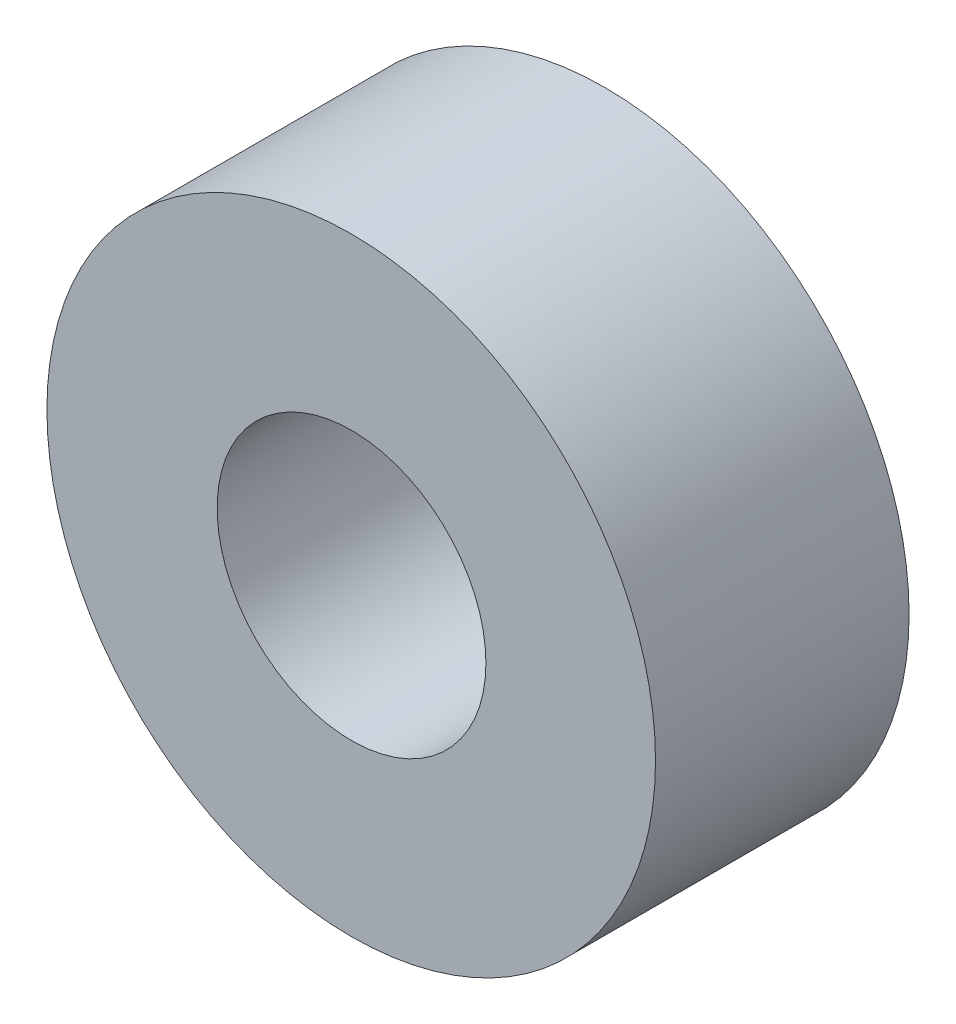
SolidWorks part; units mm, degrees
ref_plane "Front Plane" through (0, 0, 0) normal (0, 0, 1) x (1, 0, 0)
ref_plane "Top Plane" through (0, 0, 0) normal (0, 1, 0) x (1, 0, 0)
ref_plane "Right Plane" through (0, 0, 0) normal (1, 0, 0) x (0, 0, -1)
sketch "Sketch1" plane through (0, 0, 0) normal (0, 0, 1) x (1, 0, 0)
  circle A1 centre (0, 0) radius 30
extrude "Boss-Extrude1" add sketch "Sketch1" along normal blind 25
sketch "Sketch4" plane through (0, 0, 25) normal (0, 0, 1) x (1, 0, 0)
  circle A0 centre (0, 0) radius 13.2823
hole_wizard "M30 Tapped Hole3" positions "3DSketch4" profile "Sketch9" tap size "M30" standard "Gb"
sketch3d "3DSketch4"
  point P0 (0, 0, 0)
  point P3 (0.0315, -0.0033, 25)
sketch "Sketch9" plane through (0.0315, -0.0033, 25) normal (1, 0, 0) x (0, -1, 0)
  line L0 (0, 0) -> (0, 78.4614)
  line L1 (0, 78.4614) -> (13.25, 70.5)
  line L2 (13.25, 70.5) -> (13.25, 0)
  line L5 (13.25, 0) -> (0, 0)
  line L10 (0, 78.4614) -> (-13.25, 70.5) construction
  line L11 (0, -6.35) -> (0, 107.95) construction
  dimension "螺纹孔钻头直径" = 26.5
  dimension "螺纹孔钻头深度" = 70.5
  dimension "导头角度" = 118
cosmetic thread "Hole Cosmetic Thread1" parameters "D1"=25, "D2"=30
cosmetic thread "Hole Cosmetic Thread2" parameters "D1"=25, "D2"=30
